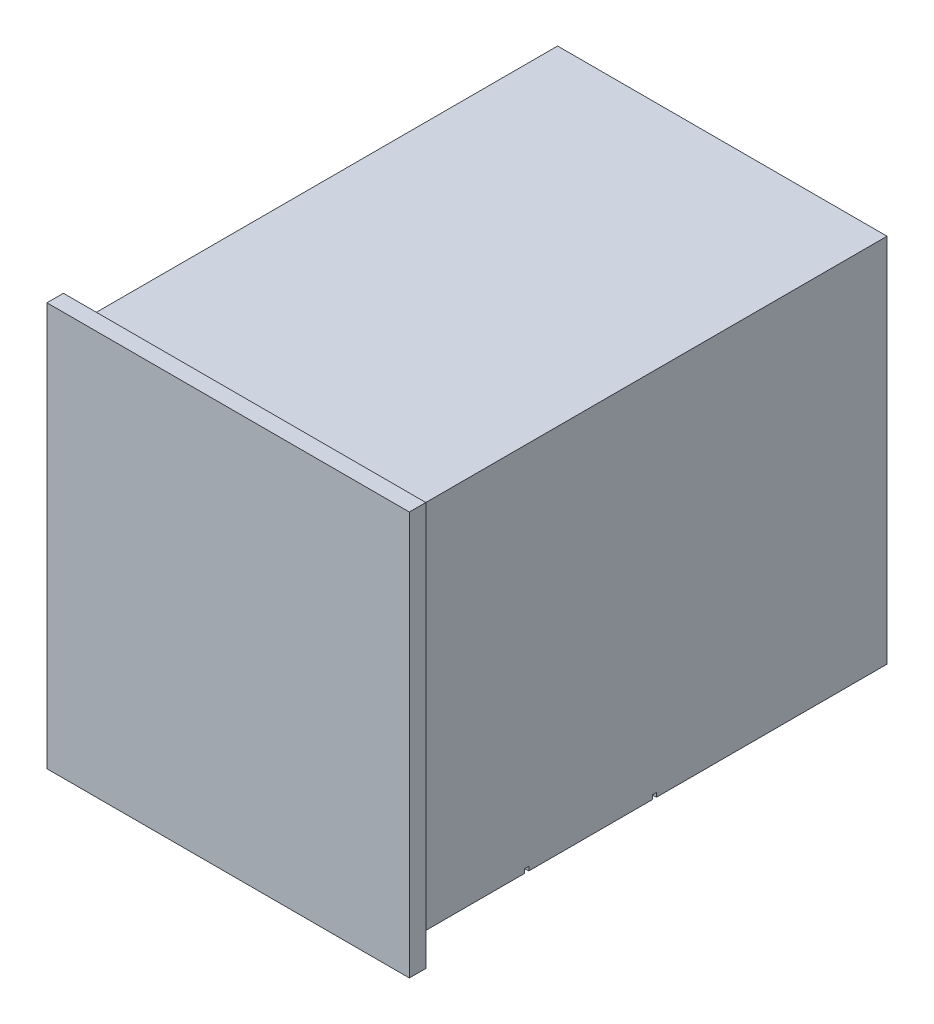
from build123d import *

# Parameters (mm, degrees)
SKETCH1_W           = 400
SKETCH1_H           = 450
BOSS_EXTRUDE1_DEPTH = 600
SKETCH2_W           = 440
SKETCH2_H           = 490
BOSS_EXTRUDE2_DEPTH = 20
SKETCH3_W           = 400
SKETCH3_H           = 5
CUT_EXTRUDE1_DEPTH  = 5
SKETCH4_W           = 400
SKETCH4_H           = 5
CUT_EXTRUDE2_DEPTH  = 5
SKETCH5_W           = 100
SKETCH5_H           = 10
BOSS_EXTRUDE3_DEPTH = 20
SKETCH6_W           = 100
SKETCH6_H           = 10
BOSS_EXTRUDE4_DEPTH = 20
SKETCH7_W           = 100
SKETCH7_H           = 10
BOSS_EXTRUDE5_DEPTH = 20
SKETCH8_W           = 90
SKETCH8_H           = 14.666116079
CUT_EXTRUDE3_DEPTH  = 500


with BuildPart() as part:
    # Sketch1 → Boss-Extrude1 (new body)
    with BuildSketch(Plane.XY):
        with Locations((200, 225)):
            Rectangle(SKETCH1_W, SKETCH1_H)
    extrude(amount=BOSS_EXTRUDE1_DEPTH)

    # Sketch2 → Boss-Extrude2 (add)
    with BuildSketch(Plane.XY.offset(600)):
        with Locations((200, 225)):
            Rectangle(SKETCH2_W, SKETCH2_H)
    extrude(amount=-BOSS_EXTRUDE2_DEPTH)

    # Sketch3 → Cut-Extrude1 (cut)
    with BuildSketch(Plane.XZ):
        with Locations((200, 437.5)):
            Rectangle(SKETCH3_W, SKETCH3_H)
    extrude(amount=-CUT_EXTRUDE1_DEPTH, mode=Mode.SUBTRACT)

    # Sketch4 → Cut-Extrude2 (cut)
    with BuildSketch(Plane.XZ):
        with Locations((200, 282.5)):
            Rectangle(SKETCH4_W, SKETCH4_H)
    extrude(amount=-CUT_EXTRUDE2_DEPTH, mode=Mode.SUBTRACT)

    # Sketch5 → Boss-Extrude3 (add)
    with BuildSketch(Plane.XZ):
        with Locations((200, 510)):
            Rectangle(SKETCH5_W, SKETCH5_H)
    extrude(amount=BOSS_EXTRUDE3_DEPTH)

    # Sketch6 → Boss-Extrude4 (add)
    with BuildSketch(Plane.XZ):
        with Locations((200, 360)):
            Rectangle(SKETCH6_W, SKETCH6_H)
    extrude(amount=BOSS_EXTRUDE4_DEPTH)

    # Sketch7 → Boss-Extrude5 (add)
    with BuildSketch(Plane.XZ):
        with Locations((200, 155)):
            Rectangle(SKETCH7_W, SKETCH7_H)
    extrude(amount=BOSS_EXTRUDE5_DEPTH)

    # Sketch8 → Cut-Extrude3 (cut)
    with BuildSketch(Plane.XY.offset(515)):
        with Locations((200, -7.666941961)):
            Rectangle(SKETCH8_W, SKETCH8_H)
    extrude(amount=-CUT_EXTRUDE3_DEPTH, mode=Mode.SUBTRACT)


solid = part.part
